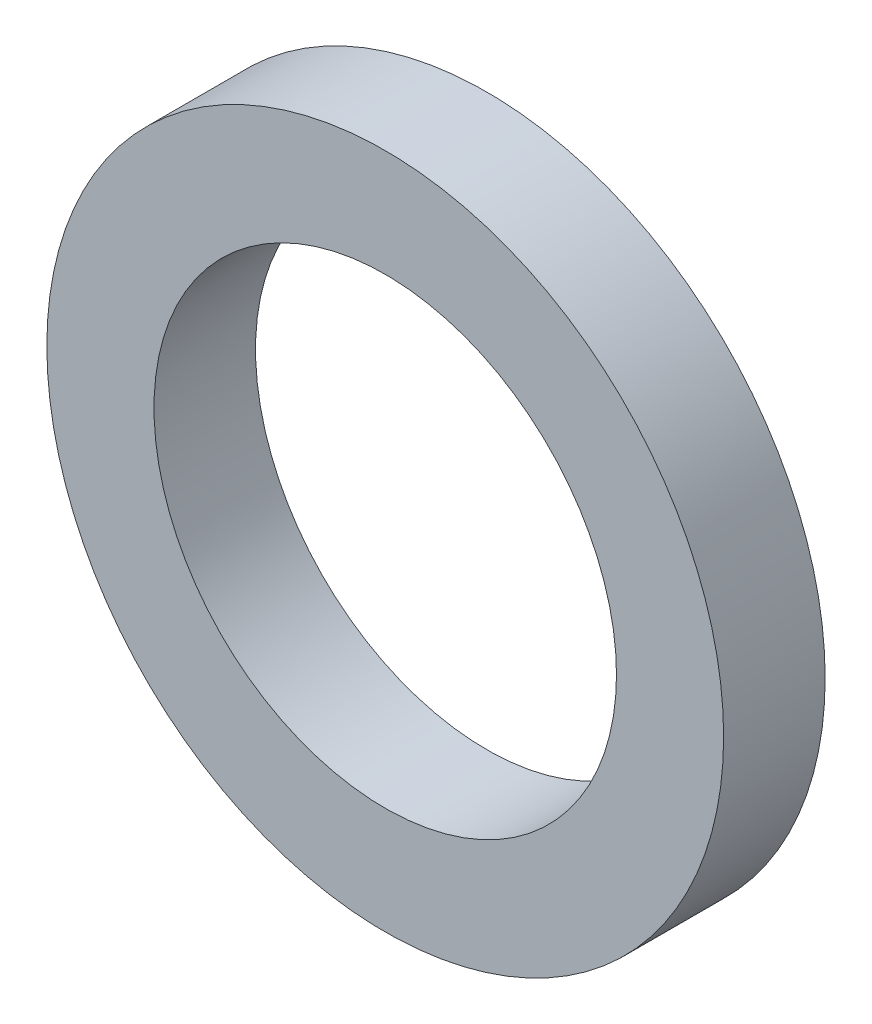
SolidWorks part; units mm, degrees
material "普通碳钢"
ref_plane "前视基准面" through (0, 0, 0) normal (0, 0, 1) x (1, 0, 0)
ref_plane "上视基准面" through (0, 0, 0) normal (0, 1, 0) x (1, 0, 0)
ref_plane "右视基准面" through (0, 0, 0) normal (1, 0, 0) x (0, 0, -1)
sketch "草图1" plane through (0, 0, 0) normal (0, 0, 1) x (1, 0, 0)
  circle A0 centre (0, 0) radius 15
  circle A1 centre (0, 0) radius 10.25
  dimension "D1" = 30
  dimension "D2" = 20.5
extrude "凸台-拉伸1" add sketch "草图1" along normal blind 4.5
